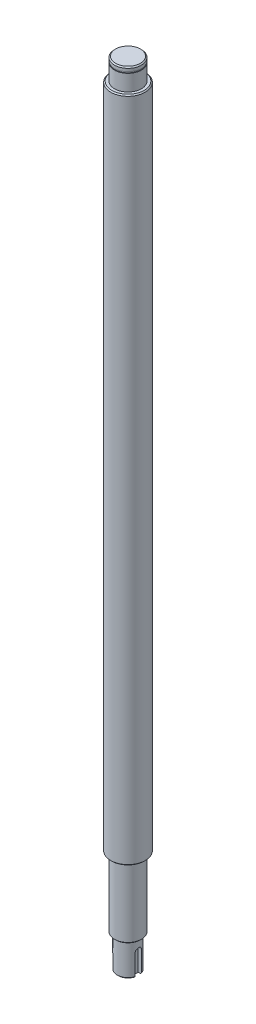
SolidWorks part; units mm, degrees
material "普通碳钢"
ref_plane "前视基准面" through (0, 0, 0) normal (0, 0, 1) x (1, 0, 0)
ref_plane "上视基准面" through (0, 0, 0) normal (0, 1, 0) x (1, 0, 0)
ref_plane "右视基准面" through (0, 0, 0) normal (1, 0, 0) x (0, 0, -1)
ref_plane "基准面2" through (0, 0, 0) normal (0, 0, -1) x (-1, 0, 0)
sketch "草图5" plane through (0, 0, 0) normal (0, 0, -1) x (-1, 0, 0)
  line L0 (-16, -294.5) -> (0, -294.5)
  line L1 (0, -294.5) -> (0, 324.5)
  line L2 (0, 324.5) -> (-16, 324.5)
  line L3 (-16, 324.5) -> (-16, -294.5)
  line L4 (0, -294.5) -> (0, 324.5) construction
  dimension "D1" = 619
  dimension "D2" = 16
revolve "旋转2" add sketch "草图5" angle 360 about L1
cosmetic thread "装饰螺纹线2" parameters "D1"=5, "D2"=27.304
sketch "草图6" plane through (0, -294.5, 0) normal (0, -1, 0) x (1, 0, 0)
  circle A0 centre (0, 0) radius 12.5
  dimension "D1" = 25
extrude "凸台-拉伸1" add sketch "草图6" along normal blind 65
cosmetic thread "装饰螺纹线1" parameters "D1"=18, "D2"=24
sketch "草图7" plane through (0, -359.5, 0) normal (0, -1, 0) x (1, 0, 0)
  circle A0 centre (0, 0) radius 10
  dimension "D1" = 20
extrude "凸台-拉伸2" add sketch "草图7" along normal blind 30
sketch "草图8" plane through (0, 324.5, 0) normal (0, 1, 0) x (1, 0, 0)
  circle A0 centre (0, 0) radius 12.5
  dimension "D1" = 25
extrude "凸台-拉伸3" add sketch "草图8" along normal blind 20
sketch "草图9" plane through (0, 0, 0) normal (0, 0, -1) x (-1, 0, 0)
  line L0 (0, 0) -> (0, 554.8462) construction
  line L2 (25.8531, 339.5) -> (11.95, 339.5)
  line L3 (25.8531, 339.5) -> (25.8531, 340.85)
  line L4 (25.8531, 340.85) -> (11.95, 340.85)
  line L5 (11.95, 339.5) -> (11.95, 340.85)
  line L6 (25.8531, 339.5) -> (11.95, 340.85) construction
  line L7 (25.8531, 340.85) -> (11.95, 339.5) construction
  line L8 (16, 324.5) -> (-16, 324.5) construction
  point P3 (18.9015, 340.175)
  dimension "D1" = 1.35
  dimension "D2" = 16.35
  dimension "D3" = 23.9
revolve "切除-旋转1" cut sketch "草图9" angle 360 about L0
chamfer "倒角1" distance 1 angle 45 5 edges at (0, -389.5, -10) (0, -359.5, -12.5) (0, -294.5, 16) (0, 324.5, 16) (0, 344.5, 12.5)
ref_plane "基准面3" through (10, 0, 0) normal (1, 0, 0) x (0, 0, -1)
sketch "草图10" plane through (10, 0, 0) normal (1, 0, 0) x (0, 0, -1)
  line L0 (0, -472.3438) -> (0, 673.0812) construction
  line L1 (0, -369.5) -> (0, -402.5535) construction
  line L2 (3, -369.5) -> (3, -402.5535)
  line L3 (-3, -369.5) -> (-3, -402.5535)
  line L4 (-9, -389.5) -> (9, -389.5) construction
  arc A0 (3, -369.5) -> (-3, -369.5) centre (0, -369.5) ccw
  arc A1 (-3, -402.5535) -> (3, -402.5535) centre (0, -402.5535) ccw
  point P5 (0, -386.0268)
  dimension "D1" = 6
  dimension "D2" = 20
extrude "切除-拉伸1" cut sketch "草图10" against normal blind 3.5
